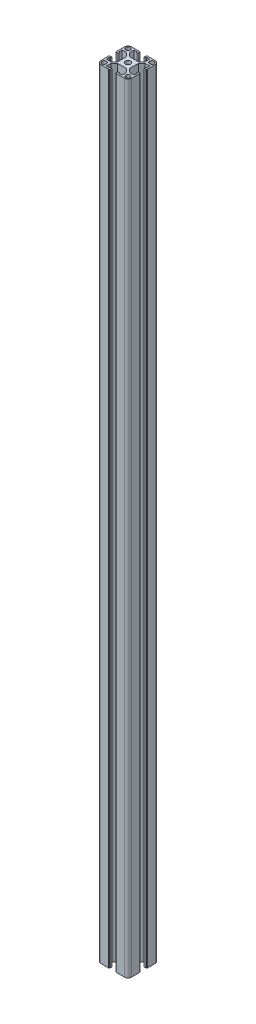
from build123d import *

# Parameters (mm, degrees)
SKETCH16_R     = 3.4
SKETCH16_R_2   = 3
MEMBER_1_DEPTH = 1013


with BuildPart() as part:
    # Sketch16 → Member 1 (new body)
    with BuildSketch(Plane(origin=(0, 0, 0), x_dir=(-1, 0, 0), z_dir=(0, 1, 0))):
        with BuildLine():
            Line((-5.1, 20), (-5.1, 19.5))
            Line((-5.1, 19.5), (-4.1, 19.5))
            Line((-4.1, 19.5), (-4.1, 17))
            Line((-4.1, 17), (-6.1, 17))
            Line((-6.1, 17), (-6.1, 18))
            Line((-6.1, 18), (-10.3, 18))
            Line((-10.3, 18), (-10.3, 12))
            Line((-10.3, 12), (-6, 7.7))
            Line((-6, 7.7), (6, 7.7))
            Line((6, 7.7), (10.3, 12))
            Line((10.3, 12), (10.3, 18))
            Line((10.3, 18), (6.1, 18))
            Line((6.1, 18), (6.1, 17))
            Line((6.1, 17), (4.1, 17))
            Line((4.1, 17), (4.1, 19.5))
            Line((4.1, 19.5), (5.1, 19.5))
            Line((5.1, 19.5), (5.1, 20))
            Line((5.1, 20), (15.5, 20))
            ThreePointArc((15.5, 20), (18.681980515, 18.681980515), (20, 15.5))
            Line((20, 15.5), (20, 5.1))
            Line((20, 5.1), (19.5, 5.1))
            Line((19.5, 5.1), (19.5, 4.1))
            Line((19.5, 4.1), (17, 4.1))
            Line((17, 4.1), (17, 6.1))
            Line((17, 6.1), (18, 6.1))
            Line((18, 6.1), (18, 10.3))
            Line((18, 10.3), (12, 10.3))
            Line((12, 10.3), (7.7, 6))
            Line((7.7, 6), (7.7, -6))
            Line((7.7, -6), (12, -10.3))
            Line((12, -10.3), (18, -10.3))
            Line((18, -10.3), (18, -6.1))
            Line((18, -6.1), (17, -6.1))
            Line((17, -6.1), (17, -4.1))
            Line((17, -4.1), (19.5, -4.1))
            Line((19.5, -4.1), (19.5, -5.1))
            Line((19.5, -5.1), (20, -5.1))
            Line((20, -5.1), (20, -15.5))
            ThreePointArc((20, -15.5), (18.681980515, -18.681980515), (15.5, -20))
            Line((15.5, -20), (5.1, -20))
            Line((5.1, -20), (5.1, -19.5))
            Line((5.1, -19.5), (4.1, -19.5))
            Line((4.1, -19.5), (4.1, -17))
            Line((4.1, -17), (6.1, -17))
            Line((6.1, -17), (6.1, -18))
            Line((6.1, -18), (10.3, -18))
            Line((10.3, -18), (10.3, -12))
            Line((10.3, -12), (6, -7.7))
            Line((6, -7.7), (-6, -7.7))
            Line((-6, -7.7), (-10.3, -12))
            Line((-10.3, -12), (-10.3, -18))
            Line((-10.3, -18), (-6.1, -18))
            Line((-6.1, -18), (-6.1, -17))
            Line((-6.1, -17), (-4.1, -17))
            Line((-4.1, -17), (-4.1, -19.5))
            Line((-4.1, -19.5), (-5.1, -19.5))
            Line((-5.1, -19.5), (-5.1, -20))
            Line((-5.1, -20), (-15.5, -20))
            ThreePointArc((-15.5, -20), (-18.681980515, -18.681980515), (-20, -15.5))
            Line((-20, -15.5), (-20, -5.1))
            Line((-20, -5.1), (-19.5, -5.1))
            Line((-19.5, -5.1), (-19.5, -4.1))
            Line((-19.5, -4.1), (-17, -4.1))
            Line((-17, -4.1), (-17, -6.1))
            Line((-17, -6.1), (-18, -6.1))
            Line((-18, -6.1), (-18, -10.3))
            Line((-18, -10.3), (-12, -10.3))
            Line((-12, -10.3), (-7.7, -6))
            Line((-7.7, -6), (-7.7, 6))
            Line((-7.7, 6), (-12, 10.3))
            Line((-12, 10.3), (-18, 10.3))
            Line((-18, 10.3), (-18, 6.1))
            Line((-18, 6.1), (-17, 6.1))
            Line((-17, 6.1), (-17, 4.1))
            Line((-17, 4.1), (-19.5, 4.1))
            Line((-19.5, 4.1), (-19.5, 5.1))
            Line((-19.5, 5.1), (-20, 5.1))
            Line((-20, 5.1), (-20, 15.5))
            ThreePointArc((-20, 15.5), (-18.681980515, 18.681980515), (-15.5, 20))
            Line((-15.5, 20), (-5.1, 20))
        make_face()
        Circle(SKETCH16_R, mode=Mode.SUBTRACT)
        with Locations((-15.556349186, 15.556349186)):
            Circle(SKETCH16_R_2, mode=Mode.SUBTRACT)
        with Locations((15.556349186, 15.556349186)):
            Circle(SKETCH16_R_2, mode=Mode.SUBTRACT)
        with Locations((15.556349186, -15.556349186)):
            Circle(SKETCH16_R_2, mode=Mode.SUBTRACT)
        with Locations((-15.556349186, -15.556349186)):
            Circle(SKETCH16_R_2, mode=Mode.SUBTRACT)
    extrude(amount=MEMBER_1_DEPTH)


solid = part.part
